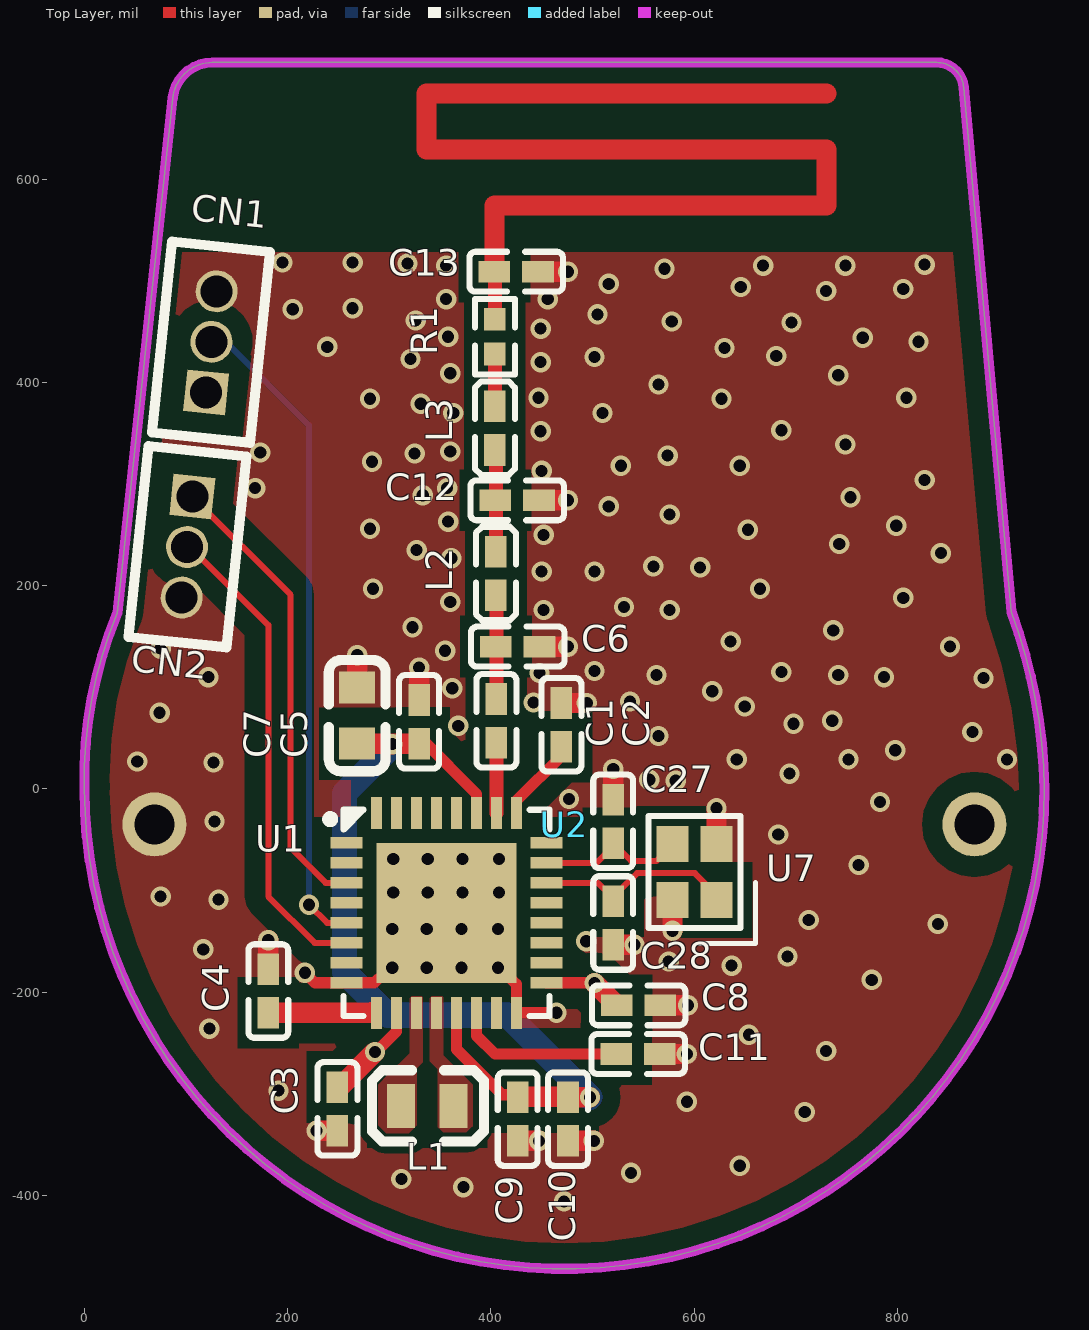
[diagram p0: Top Layer view]
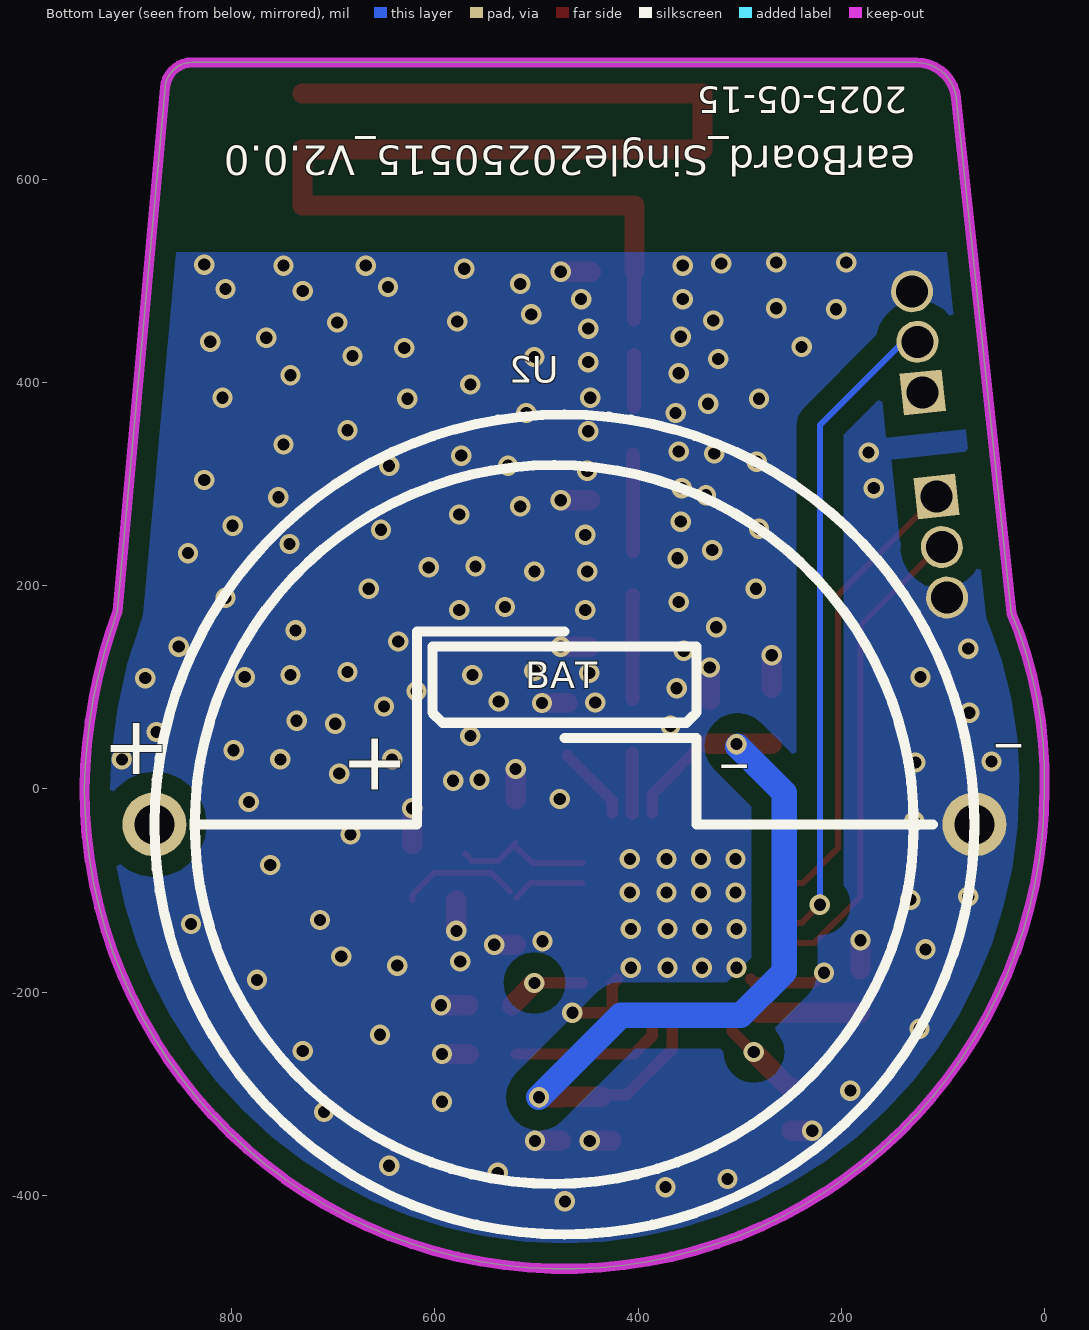
[diagram p1: Bottom Layer view, seen from below]
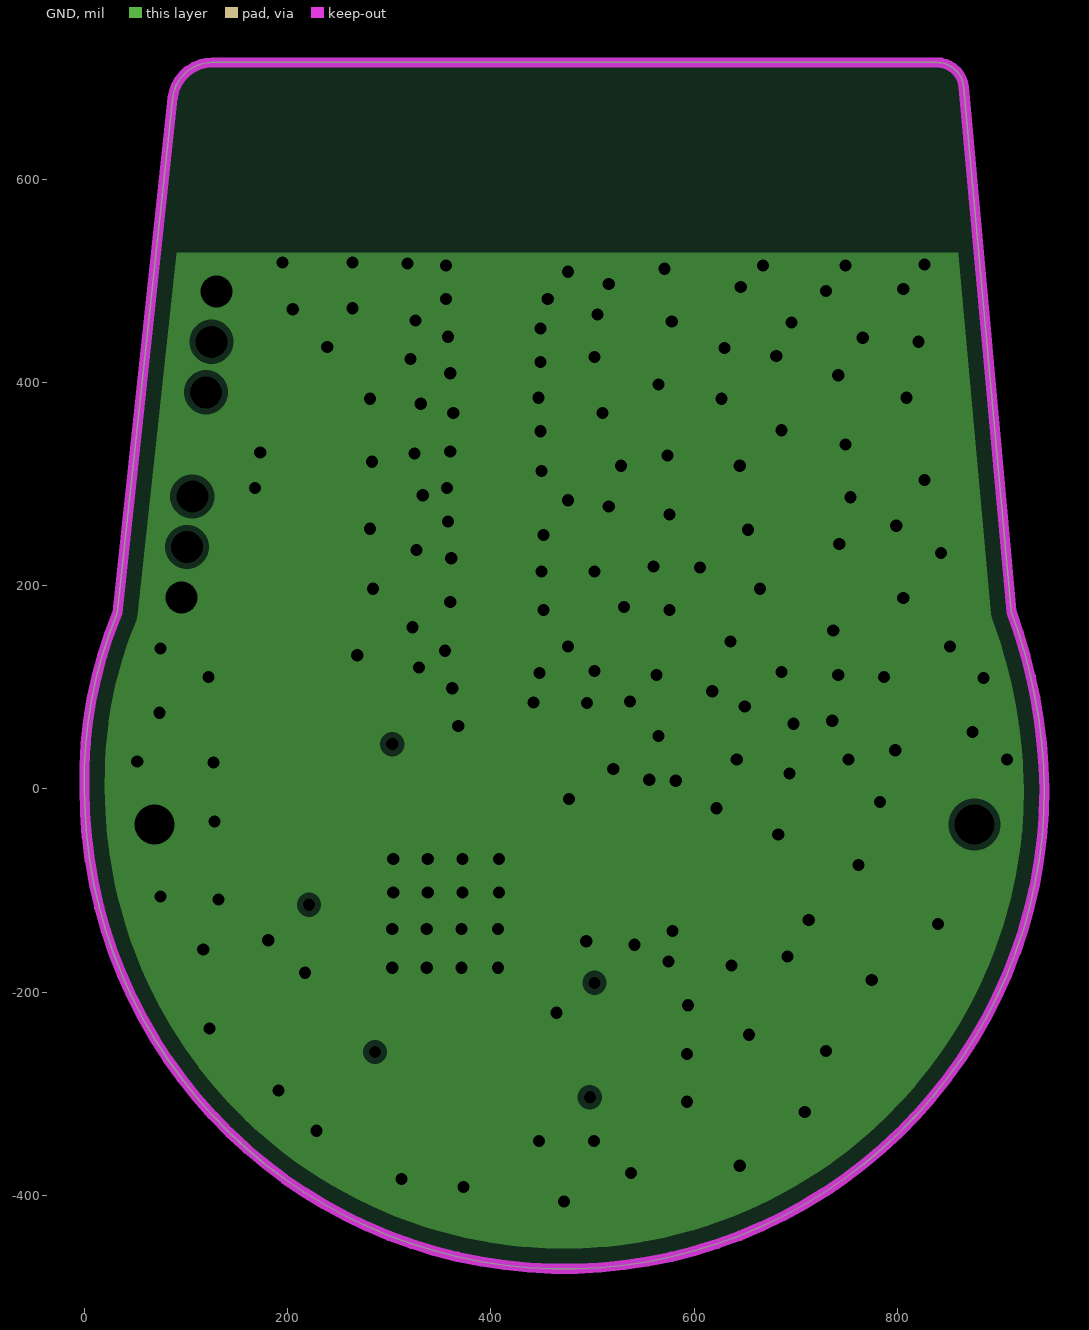
[diagram p2: GND, clearances drawn from the general rule]
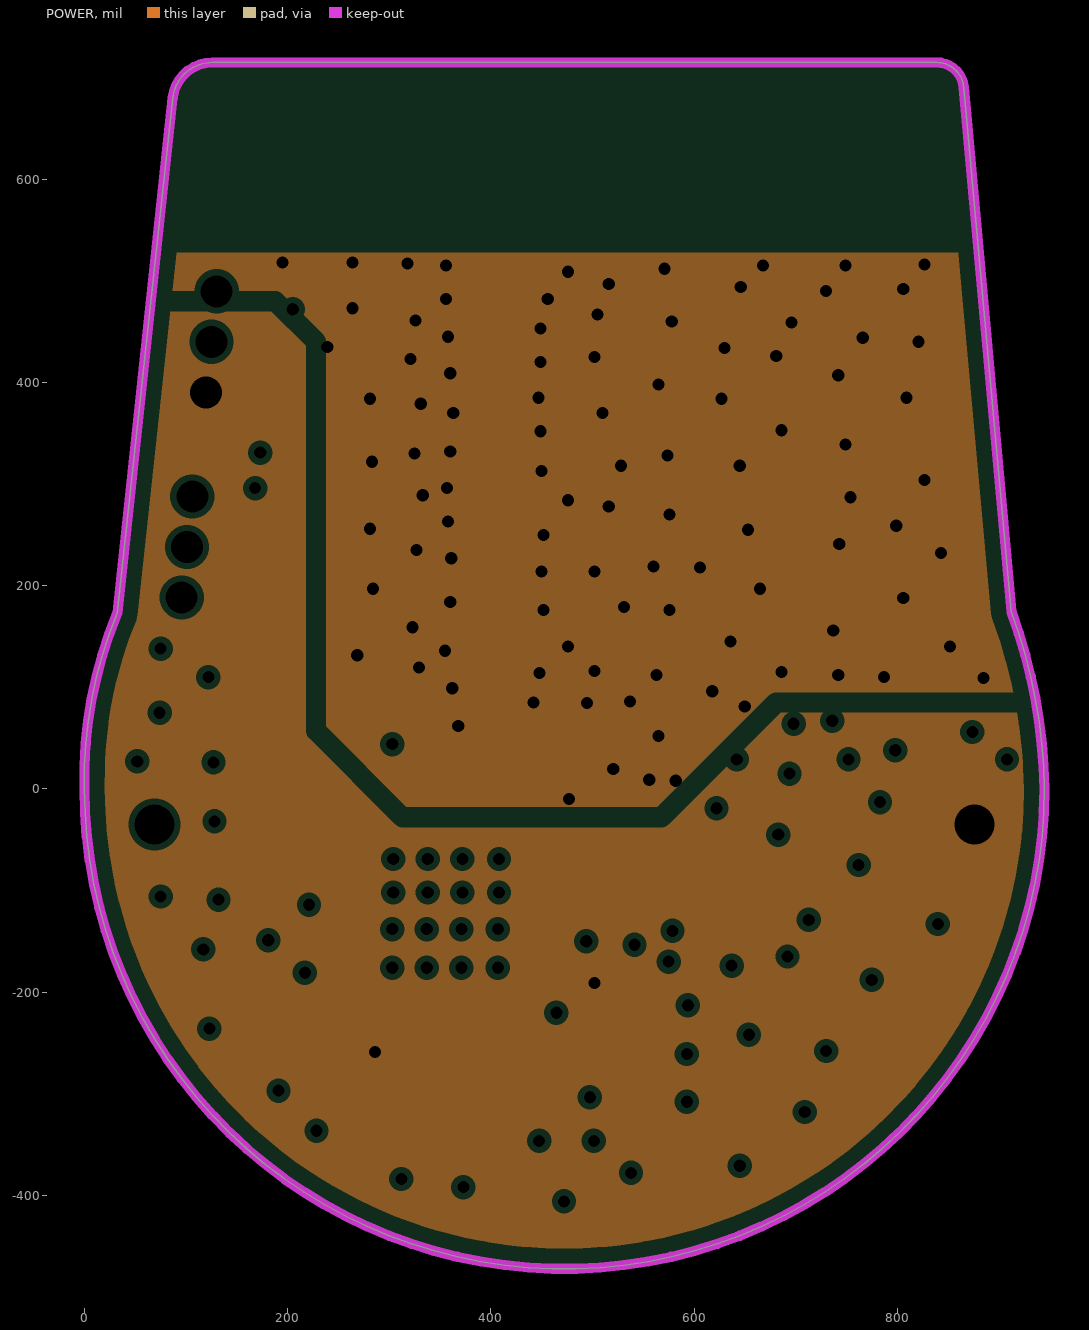
[diagram p3: POWER, clearances drawn from the general rule]
# Altium PCB MISC79017.PcbDoc
Units mil, origin at the board's own origin, x right, y up, seen from the top; angles counter-clockwise.
Board outline 944.88 x 1187.29 mil, 4 copper layers (Top Layer, GND, POWER, Bottom Layer); 24 components, 18 nets, 83 pads, 177 vias.

## Layer stack, top to bottom (the 12.6 mil dielectric is the usual default, probably not edited)
Top Layer: signal copper 1.4
Dielectric: core 12.6, FR-4, Dk 4.8
GND: plane copper 1.4, net GND
Dielectric: prepreg 12.6, FR-4, Dk 4.8
POWER: plane copper 1.4, net (Multiple Nets)
Dielectric: core 12.6, FR-4, Dk 4.8
Bottom Layer: signal copper 1.4

## Board outline
0,0 cw(c423.07,10.33) 32.44,173.13 86.87,679.83 cw(c126.01,675.63) 126.01,715 838.85,715 cw(c838.85,688.29) 865.48,690.34 912.44,174.28 912.44,174.29 cw(c411.43,-9.14) 944.88,0 cw(c472.44,0)

## Design rules (kind name [scope] priority, off if disabled: settings)
Clearance Clearance_1 [inpolygon] p1: gap=6
Clearance [All] p2: gap=6
HoleToHoleClearance [All] p1: gap=0 allowstackedmicrovias=TRUE
MinimumSolderMaskSliver [All] p1: minsoldermaskwidth=0
PlaneClearance [All] p1: clearance=6
PlaneConnect [All] p1: planeconnectstyle=Direct reliefexpansion=20 reliefentries=4 reliefconductorwidth=10 reliefairgap=10
PolygonConnect [All] p1: connectstyle=Direct reliefconductorwidth=10 reliefentries=4 polygonreliefangle="90 Angle"
RoutingVias [All] p1: holewidth=12 width=20 viastyle="Through Hole" minholewidth=12 minwidth=20 maxholewidth=12 maxwidth=20
SilkToSilkClearance [All] p1: silktosilkclearance=0
SilkscreenOverComponentPads [All] p1: minsilkscreentomaskgap=0
SolderMaskExpansion [All] p1: expansion=4
Width [All] p1: maxlimit=40 minlimit=6 preferedwidth=6
22 further rules are at their usual default settings.

## Components (designator, comment, footprint, x,y, rotation, side; value= is the part's Value field where it differs from the comment)
C1 "220pF" C0402 405.46,67 r90 top
C2 "1uF" C0402 469.46,63 r270 top
C3 "1uF" C0402 249,-315 r90 top
C4 "1uF" C0402 181,-199 r270 top
C5 "1uF" C0402 329.46,66 r270 top
C6 "2pF" C0402 426.46,140 r180 top
C7 "0.1uF" C0603 268.46,72 r270 top
C8 "1uF" C0402 545.46,-213 r0 top
C9 "2.2uF" C0402 426.46,-325 r90 top
C10 "0.1uF" C0402 476,-325 r90 top
C11 "1uF" C0402 545,-261 r180 top
C12 "2pF" C0402 426,284 r180 top
C13 "2pF" C0402 425,509 r180 top
C27 "12pF" C0402 520.46,-32 r90 top
C28 "12pF" C0402 520.46,-132 r270 top
CN1 "" HDR-TH_3P-P1.27-V-M-A 125,440 r84 top
CN2 "" HDR-TH_3P-P1.27-V-M-A 101,238 r264 top
L1 "4.7uH" IND-SMD_L1.8-W1.2 337.46,-312 r0 top
L2 "2.4nH" L0402 405,212 r90 top
L3 "2.4nH" L0402 404,355 r90 top
R1 "" R0402 404,445 r90 top
U1 "TLSR8355F512ET32" TQFN-32_L5.0-W5.0-P0.50-BL-EP3.5 356.46,-122 r270 top locked
U2 "Q&J CR2032 20-6*9" BAT-TH_CR2032 472.44,-35 r180 top locked
U7 "24MHz" JWT1238 600.46,-82 r90 top

## Footprints (in the part's own frame and the unit in brackets; to place one, negate y for a bottom-side part, rotate by r counter-clockwise, add the part's x,y. Pads: shape width x height; smd on the part's side, far side on the other; paste and mask are expansions set on the pad)
BAT-TH_CR2032 [mm]
  round 1.6 hole 1: 1(-10.25,0) 2(10.25,0)
C0402 [mm]
  rect 0.79x0.54 smd paste-100 mask+0.051: 1(-0.545,0) 2(0.545,0)
  silkscreen extent -1.17,-0.5 1.17,0.5
C0603 [mm]
  rect 0.8x0.9 smd: 1(-0.7,0) 2(0.7,0)
  silkscreen extent -1.39,-0.71 1.39,0.71
HDR-TH_3P-P1.27-V-M-A [mm]
  rect 1.05x1.05 hole 0.8: 1(-1.27,0)
  round 1.05 hole 0.8: 2(0,0) 3(1.27,0)
  silkscreen extent -2.41,-1.22 2.39,1.24
IND-SMD_L1.8-W1.2 [mm]
  rect 0.7x1.1 smd: 1(-0.653,0) 2(0.653,0)
  silkscreen extent -1.38,-0.89 1.41,0.89
JWT1238 [mm]
  rect 0.9x0.8 smd: 1(-0.7,-0.55) 2(0.7,-0.55) 3(0.7,0.55) 4(-0.7,0.55)
  silkscreen extent -1.78,-1.52 1.4,1.15
L0402 [mm]
  rect 0.79x0.54 smd paste-100 mask+0.051: 1(-0.545,0) 2(0.545,0)
  silkscreen extent -1.17,-0.5 1.17,0.5
R0402 [mm]
  rect 0.566x0.54 smd paste-100 mask+0.051: 1(-0.433,0) 2(0.433,0)
  silkscreen extent -0.94,-0.5 0.94,0.5
TQFN-32_L5.0-W5.0-P0.50-BL-EP3.5 [mm]
  rect 0.28x0.8 smd paste-100 mask+0.051: 1(-1.75,-2.5) 2(-1.25,-2.5) 3(-0.75,-2.5) 4(-0.25,-2.5) 5(0.25,-2.5) 6(0.75,-2.5) 7(1.25,-2.5) 8(1.75,-2.5) 17(1.75,2.5) 18(1.25,2.5) 19(0.75,2.5) 20(0.25,2.5) 21(-0.25,2.5) 22(-0.75,2.5) 23(-1.25,2.5) 24(-1.75,2.5)
  rect 0.8x0.28 smd paste-100 mask+0.051: 9(2.5,-1.75) 10(2.5,-1.25) 11(2.5,-0.75) 12(2.5,-0.25) 13(2.5,0.25) 14(2.5,0.75) 15(2.5,1.25) 16(2.5,1.75) 25(-2.5,1.75) 26(-2.5,1.25) 27(-2.5,0.75) 28(-2.5,0.25) 29(-2.5,-0.25) 30(-2.5,-0.75) 31(-2.5,-1.25) 32(-2.5,-1.75)
  rect 3.5x3.5 smd paste-100 mask+0.051: 33(0,0)
  silkscreen extent -2.58,-3.01 2.58,2.58

## Part data
C1: library part CC0402KRX7R9BB221
C2 C3 C4 C5 C8 C9 C10 C11: library part CL05A105KA5NQNC
C6 C12 C13: library part CC0402CRNPO9BN2R0
C7: library part CAP_0603
C27 C28: library part 0402CG120J500NT
CN1 CN2: library part 3Pin_1.27___
L1: library part SLC1608F4R7KTT
L2 L3: library part LQG15HH2N4S02D
R1: library part SCR0402J0R
U7: library part JWT1238

## Via types
v1: diameter 20, hole 12, Top Layer to Bottom Layer, 177 vias

## Nets (pads, with @x,y where several pads share a name; then routed paths per layer and width w, separated by ;. In a path a pad name is that pad's centre, name@x,y a point inside that pad or via, vN(x,y) a via of type N, cw(c..) or ccw(c..) an arc to the next point about the centre after c; other vN are vias at no path point)
ANT: C1.1 U1.26 | length 57.9
  Top Layer w13.75: U1.26 C1.1@405.67,34.33
ANTENNA: C13.2 R1.2 | length 1331.3
  Top Layer w13.75: R1.2 C13.2@404,504
  Top Layer w19.68: C13.2 403.54,573.96 730.31,573.96 730.31,629.08 336.61,629.08 336.61,684.2 730.31,684.2
GND: C2.1 C3.1 C4.1 C5.1 C6.1 C7.1 C8.2 C9.1 C10.1 C11.1 C12.1 C13.1 C27.2 C28.2 CN1.3 CN2.3 U1.8 U1.16 U1.33 U2.2 U7.2 U7.4 | length 593.6
  Top Layer w11: v1(217,-181) 226.9,-190.9 U1.8 285.1,-190.9 U1.33@289,-187 ; U1.33@420,-187 425.36,-192.36 425.36,-202 U1.16 v1(464.58,-220.42)
  Top Layer w20: C4.1 v1(181,-149) ; v1(228.46,-336.46) C3.1 ; C7.1 v1(268.46,131.54) ; C5.1 v1(329.46,119.46) ; C9.1 v1(447.54,-346.46) ; C13.1 v1(476,509) ; C12.1 v1(476,284) ; C6.1 v1(476,140) ; C2.1 v1(494.54,84.46) ; C10.1 v1(501.46,-346.46) ; C28.2 v1(541.46,-153.46) ; C27.2 v1(520.46,19.46) ; C11.1 v1(593,-261) ; C8.2 v1(594,-213) ; v1(578.8,-139.8) U7.4 ; U7.2 v1(622.12,-19.12)
  other v1: 472,-406 373,-392 312,-384 538,-378 645,-371 709,-318 593,-308 191,-297 730,-258 654,-242 123,-236 775,-188 303,-176 337,-176 371,-176 407,-176 637,-174 575,-170 692,-165 117,-158 494,-150 303,-138 337,-138 371,-138 407,-138 840,-133 713,-129 132,-109 75,-106 304,-102 338,-102 372,-102 408,-102 762,-75 304,-69 338,-69 372,-69 408,-69 683,-45 128,-32 783,-13 477,-10 582,8 556,9 694,15 127,26 52,27 642,29 752,29 908,29 798,38 565,52 874,56 368,62 698,64 736,67 74,75 650,81 442,85 537,86 618,96 362,99 885,109 122,110 787,110 563,112 742,112 448,114 686,115 502,116 355,136 75,138 852,140 636,145 737,156 323,159 452,176 576,176 531,179 360,184 806,188 284,197 665,197 450,214 502,214 606,218 560,219 361,227 843,232 327,235 743,241 452,250 653,255 281,256 799,259 358,263 576,270 516,278 754,287 333,289 168,296 357,296 827,304 450,313 528,318 645,318 283,322 574,328 325,330 173,331 360,332 749,339 449,352 686,353 363,370 510,370 331,379 281,384 627,384 447,385 809,385 565,398 742,407 360,409 449,420 321,423 502,425 681,426 630,434 239,435 821,440 766,444 358,445 449,453 696,459 578,460 326,461 505,467 205,472 264,473 356,482 456,482 730,490 806,492 646,494 516,497 571,512 356,515 668,515 749,515 827,516 318,517 195,518 264,518
NetC1_2: C1.2 C6.2 L2.1 | length 102.7
  Top Layer w13.75: L2.1@405,191 405.46,190.54 C1.2
NetC4_2: C4.2 U1.9 | length 101.2
  Top Layer w20: C4.2 281.54,-220.46 282,-220
NetC12_2: C12.2 L2.2 L3.1 | length 95.5
  Top Layer w13.75: L2.2 L3.1@405,329
NetL1_1: L1.1 U1.11
NetL1_2: L1.2 U1.12
NetL3_2: L3.2 R1.1 | length 50.5
  Top Layer w13.75: L3.2 R1.1@404,427
RX: CN2.2 U1.6 | length 456.2
  Top Layer w6: CN2.2@115,227 181,161 181,-106 226.53,-151.53 U1.6
TL_1V4: C5.2 C7.2 C9.2 C10.2 U1.13 U1.27 | length 876.2
  Top Layer w11: C5.2@330,48 333,48 385.99,-4.99 U1.27 ; U1.13 366.3,-256.3 411,-301 C9.2@429,-301 ; C9.2@428.5,-301.5 429,-302 C9.2@436,-302
  Top Layer w20: C7.2 v1@303,44.44 ; v1(303,44) v1@303,44.44 ; C5.2@329.56,44.44 v1@303,44.44 ; C9.2@436,-303 C10.2@474,-303 ; C10.2 v1(497.54,-303.54)
  Bottom Layer w25: v1@302,42 256,-4 256,-180 299,-223 417,-223 v1(497.54,-303.54)
TL_RST: C2.2 U1.25 | length 75.1
  Top Layer w11: U1.25 425.36,-11.64 C2.2@470,33
TL_SWS_A7: CN1.2 U1.5 | length 631
  Top Layer w6: v1(221,-114) 238.84,-131.84 U1.5
  Bottom Layer w6: CN1.2@140,439 221,358 221,-92 v1(221,-114)
TL_VDD3: C3.2 C8.1 CN1.1 U1.10 U1.17 U2.1 | length 214.9
  Top Layer w11: C3.2@255,-291 307.25,-238.75 U1.10 ; U1.17 v1@495.1,-190.9
  Top Layer w20: C3.2 251.46,-293.54 v1(286,-259) ; v1(502,-191) C8.1
TL_XC1: C27.1 U1.23 U7.3 | length 128.7
  Top Layer w6: U1.23 504.21,-72.79 C27.1@518,-59 ; C27.1 538,-71 539.03,-71 ; 539.17,-70.86 539.03,-71 ; U7.3@570,-64 563.14,-70.86 554.35,-70.86 554.21,-71 539.03,-71
TL_XC2: C28.1 U1.22 U7.1 | length 189
  Top Layer w6: U1.22 505.47,-92.47 C28.1@520,-107 ; C28.1@526,-101 544,-83 559.18,-83 559.33,-82.86 568.11,-82.86 600.86,-82.86 622.11,-104.11 U7.1
TX: CN2.1 U1.3 | length 455.1
  Top Layer w6: CN2.1 203,190.95 203,-58 237.47,-92.47 U1.3
VDD_1V8: C11.2 U1.14 | length 164
  Top Layer w11: U1.14 385.99,-242.99 404,-261 C11.2@520,-261
pads on no net: U1.1 U1.2 U1.4 U1.7 U1.15 U1.18 U1.19 U1.20 U1.21 U1.24 U1.28 U1.29 U1.30 U1.31 U1.32

## Polygon pours and split planes (outlines as drawn)
GND on Top Layer "Bottom Layer-No Net" (solid, remove dead copper): -136,693 -136,-347 21,-504 88,-571 545,-571 900,-571 1043,-428 1138,-333 1138,-80 1138,783 995,926 963,958 711,958 -5,958 -94,869 -132,831 -132,693
NetL1_2 on Top Layer "Bottom Layer-No Net" (solid, remove dead copper): 340,-221 340,-268 345,-273 348,-276 348,-287 348,-333 351,-336 353,-338 356,-338 376,-338 380,-334 382,-332 382,-329 382,-291 366,-275 353,-262 353,-228 353,-205 352,-204 347,-204 342,-204 341,-205 340,-206 340,-220
NetL1_1 on Top Layer "Bottom Layer-No Net" (solid, remove dead copper): 320,-221 320,-237 320,-260 299,-281 289,-291 289,-312 289,-331 293,-335 297,-339 299,-339 319,-339 324,-334 327,-331 327,-288 327,-275 331,-271 333,-269 333,-235 333,-205 332,-204 331,-204 322,-204 321,-205 320,-206 320,-221
GND on Bottom Layer "Bottom Layer-No Net" (solid, remove dead copper): -107,667 -107,-329 21,-457 129,-565 589,-565 823,-565 963,-425 1049,-339 1049,-214 1049,830 950,929 918,961 733,961 36,961 -56,869 -110,815 -110,683
GND on GND (split plane): 892.43,172.46 892.54,171.88 892.57,171.28 892.68,170.83 892.73,170.36 893,169.49 893.17,168.59 893.39,168.04 893.54,167.46 893.82,166.86 899.83,149.55 905.68,130.26 910.77,110.74 915.09,91.05 918.64,71.2 921.4,51.22 923.38,31.15 924.56,11.02 924.79,-0.35 924.82,-0.35 924.86,-0.79 924.49,-18.7 923.33,-37.36 921.4,-55.96 918.71,-74.47 915.25,-92.85 911.03,-111.07 906.07,-129.1 900.36,-146.91 893.93,-164.46 886.77,-181.74 878.91,-198.71 870.35,-215.34 861.11,-231.6 851.21,-247.46 840.66,-262.9 829.48,-277.89 817.69,-292.41 805.31,-306.43 792.36,-319.92 778.87,-332.87 764.85,-345.25 750.33,-357.04 735.34,-368.22 719.9,-378.77 704.04,-388.67 687.78,-397.91 671.15,-406.47 654.18,-414.33 636.91,-421.49 619.35,-427.92 601.54,-433.63 583.51,-438.59 565.29,-442.81 546.91,-446.27 528.4,-448.96 509.8,-450.89 491.14,-452.05 472.44,-452.44 453.74,-452.05 435.08,-450.89 416.48,-448.96 397.97,-446.27 379.59,-442.81 361.37,-438.59 343.34,-433.63 325.53,-427.92 307.98,-421.49 290.7,-414.33 273.73,-406.47 257.1,-397.91 240.84,-388.67 224.98,-378.77 209.54,-368.22 194.55,-357.04 180.03,-345.25 166.01,-332.87 152.52,-319.92 139.57,-306.43 127.19,-292.41 115.4,-277.89 104.23,-262.9 93.68,-247.46 83.77,-231.6 74.53,-215.34 65.98,-198.71 58.11,-181.74 50.95,-164.46 44.52,-146.91 38.81,-129.1 33.85,-111.07 29.63,-92.85 26.17,-74.47 23.48,-55.96 21.55,-37.36 20.39,-18.7 20.02,-0.79 20.1,0 20.05,0.49 20.09,0.49 19.88,10.33 20.26,27.92 21.41,45.47 23.33,62.96 26,80.34 29.44,97.6 33.62,114.68 38.54,131.57 44.19,148.23 50.49,164.42 50.84,165.04 50.96,165.41 50.99,165.4 51.01,165.44 51.27,166.3 51.62,167.13 51.79,167.96 52.06,168.78 52.09,169 52.15,169.21 52.24,170.11 52.42,170.98 90.77,528 860.07,528
TL_VDD3 on POWER (split plane): 217.91,435.82 217.91,57 218.26,54.39 219.27,51.96 220.87,49.87 305.87,-35.13 307.96,-36.74 308.67,-37.03 310.39,-37.74 313,-38.09 568,-38.09 570.61,-37.74 573.04,-36.74 575.13,-35.13 685.18,74.91 917.97,74.91 918.64,71.2 921.4,51.22 923.38,31.15 924.56,11.02 924.79,-0.35 924.82,-0.35 924.86,-0.79 924.49,-18.7 923.33,-37.36 921.4,-55.96 918.71,-74.47 915.25,-92.85 911.03,-111.07 906.07,-129.1 900.36,-146.91 893.93,-164.46 886.77,-181.74 878.91,-198.71 870.35,-215.34 861.11,-231.6 851.21,-247.46 840.66,-262.9 829.48,-277.89 817.69,-292.41 805.31,-306.43 792.36,-319.92 778.87,-332.87 764.85,-345.25 750.33,-357.04 735.34,-368.22 719.9,-378.77 704.04,-388.67 687.78,-397.91 671.15,-406.47 654.18,-414.33 636.91,-421.49 619.35,-427.92 601.54,-433.63 583.51,-438.59 565.29,-442.81 546.91,-446.27 528.4,-448.96 509.8,-450.89 491.14,-452.05 472.44,-452.44 453.74,-452.05 435.08,-450.89 416.48,-448.96 397.97,-446.27 379.59,-442.81 361.37,-438.59 343.34,-433.63 325.53,-427.92 307.98,-421.49 290.7,-414.33 273.73,-406.47 257.1,-397.91 240.84,-388.67 224.98,-378.77 209.54,-368.22 194.55,-357.04 180.03,-345.25 166.01,-332.87 152.52,-319.92 139.57,-306.43 127.19,-292.41 115.4,-277.89 104.23,-262.9 93.68,-247.46 83.77,-231.6 74.53,-215.34 65.98,-198.71 58.11,-181.74 50.95,-164.46 44.52,-146.91 38.81,-129.1 33.85,-111.07 29.63,-92.85 26.17,-74.47 23.48,-55.96 21.55,-37.36 20.39,-18.7 20.02,-0.79 20.1,0 20.05,0.49 20.09,0.49 19.88,10.33 20.26,27.92 21.41,45.47 23.33,62.96 26,80.34 29.44,97.6 33.62,114.68 38.54,131.57 44.19,148.23 50.49,164.42 50.84,165.04 50.96,165.41 50.99,165.4 51.01,165.44 51.27,166.3 51.62,167.13 51.79,167.96 52.06,168.78 52.09,169 52.15,169.21 52.24,170.11 52.42,170.98 84.53,469.91 183.82,469.91
GND on POWER (split plane): 892.43,172.46 892.54,171.88 892.57,171.28 892.68,170.83 892.73,170.36 893,169.49 893.17,168.59 893.39,168.04 893.54,167.46 893.82,166.86 899.83,149.55 905.68,130.26 910.77,110.74 914.21,95.09 681,95.09 678.39,94.74 677.68,94.45 675.96,93.74 673.87,92.13 563.82,-17.91 317.18,-17.91 238.09,61.18 238.09,440 237.74,442.61 237.45,443.32 236.74,445.04 235.13,447.13 195.13,487.13 193.04,488.74 190.61,489.74 188,490.09 86.7,490.09 90.77,528 860.07,528

## Keep-outs
Keep-Out Layer:
  the board outline again, w10

## Other copper
GND (plane layer: these items are gaps in the copper):
  rectangle: 75,528 867,731
POWER (plane layer: these items are gaps in the copper):
  rectangle: 75,528 878,731
  lines w20: 71,480 188,480 228,440 228,57 313,-28 568,-28 681,85 932,85
Multi-Layer:
  pour cut-out: 6,750 6,562 40,528 920,528 952,560 952,795 895,852 75,852 7,784 7,751

## Silkscreen, mask and mechanical layers (free items; w line width, h text height)
Bottom Overlay:
  text "2025-05-15" at 135,700 h45 r180
  text "earBoard_Single20250515_V2.0.0" at 127,643 h50 r180